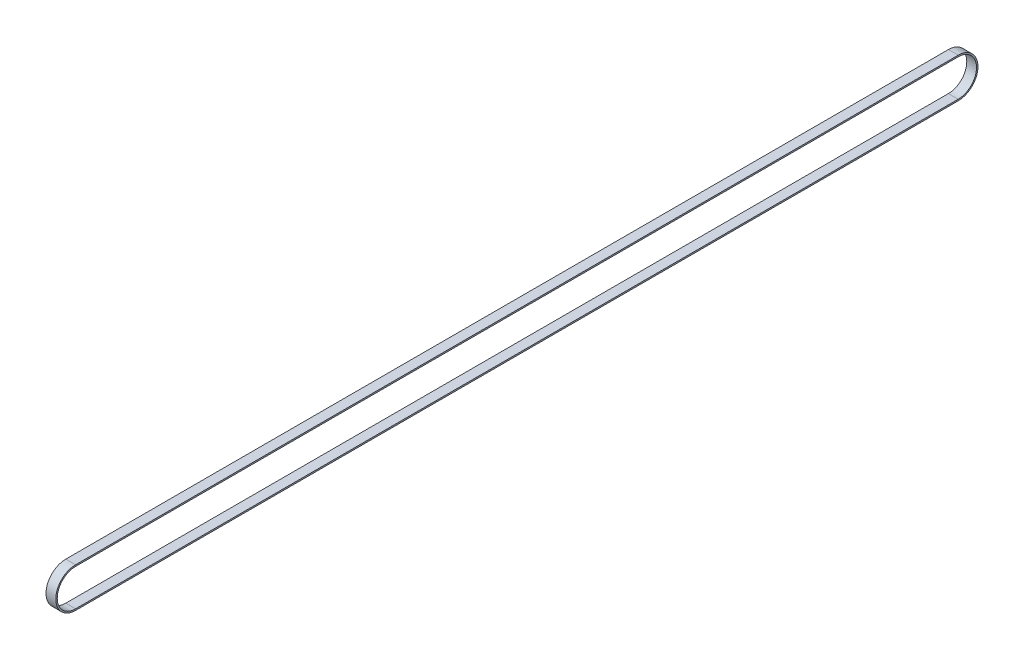
SolidWorks part; units mm, degrees
material "聚脂树脂"
ref_plane "前视基准面" through (0, 0, 0) normal (0, 0, 1) x (1, 0, 0)
ref_plane "上视基准面" through (0, 0, 0) normal (0, 1, 0) x (1, 0, 0)
ref_plane "右视基准面" through (0, 0, 0) normal (1, 0, 0) x (0, 0, -1)
sketch "草图2" plane through (0, 0, 0) normal (1, 0, 0) x (0, 0, -1)
  line L0 (0, 57.295) -> (-2710, 57.295)
  line L6 (-2710, -57.295) -> (0, -57.295)
  arc A0 (0, -57.295) -> (0, 57.295) centre (0, 0) ccw
  arc A1 (-2710, 57.295) -> (-2710, -57.295) centre (-2710, 0) ccw
  dimension "D2" = 114.59
  dimension "D7" = 2710
extrude "拉伸-薄壁1" add sketch "草图2" along normal mid plane 30 thin
